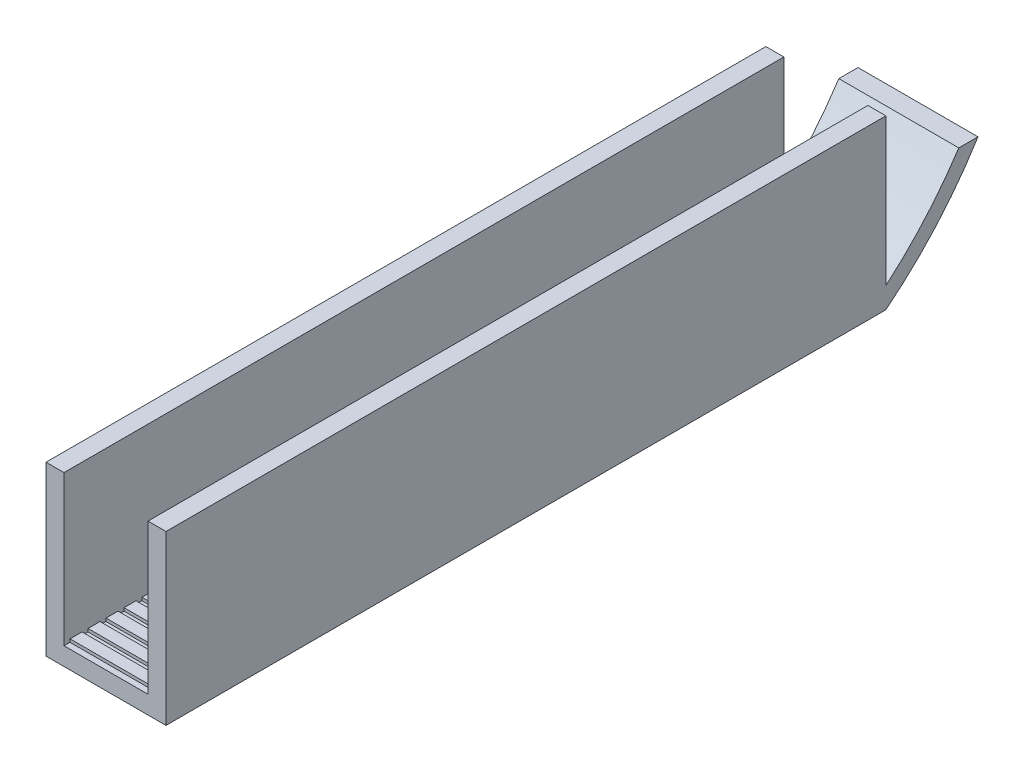
SolidWorks part; units mm, degrees
ref_plane "Front" through (0, 0, 0) normal (0, 0, 1) x (1, 0, 0)
ref_plane "Top" through (0, 0, 0) normal (0, 1, 0) x (1, 0, 0)
ref_plane "Right" through (0, 0, 0) normal (1, 0, 0) x (0, 0, -1)
sketch "Sketch1" plane through (0, 0, 0) normal (0, 0, 1) x (1, 0, 0)
  line L1 (0, 0) -> (-200, 0)
  line L2 (0, 0) -> (0, 30)
  line L3 (0, 30) -> (-200, 30)
  line L4 (-200, 0) -> (-200, 30)
  dimension "D1" = 200
  dimension "D2" = 30
extrude "Boss-Extrude1" add sketch "Sketch1" along normal blind 1200
sketch "Sketch2" plane through (0, 30, 0) normal (0, 1, 0) x (1, 0, 0)
  line L0 (-200, -1200) -> (-200, 0) construction
  line L1 (0, 0) -> (-200, 0)
  line L2 (0, 0) -> (0, -20)
  line L3 (0, -20) -> (-200, -20)
  line L4 (-200, 0) -> (-200, -20)
  line L5 (0, -50) -> (-200, -50)
  line L6 (0, -30) -> (-200, -30)
  line L7 (0, -30) -> (0, -50)
  line L8 (-200, -30) -> (-200, -50)
  line L9 (0, -80) -> (-200, -80)
  line L10 (0, -60) -> (-200, -60)
  line L11 (0, -60) -> (0, -80)
  line L12 (-200, -60) -> (-200, -80)
  line L13 (0, -110) -> (-200, -110)
  line L14 (0, -90) -> (-200, -90)
  line L15 (0, -90) -> (0, -110)
  line L16 (-200, -90) -> (-200, -110)
  line L17 (0, -140) -> (-200, -140)
  line L18 (0, -120) -> (-200, -120)
  line L19 (0, -120) -> (0, -140)
  line L20 (-200, -120) -> (-200, -140)
  line L21 (0, -170) -> (-200, -170)
  line L22 (0, -150) -> (-200, -150)
  line L23 (0, -150) -> (0, -170)
  line L24 (-200, -150) -> (-200, -170)
  line L25 (0, -200) -> (-200, -200)
  line L26 (0, -180) -> (-200, -180)
  line L27 (0, -180) -> (0, -200)
  line L28 (-200, -180) -> (-200, -200)
  line L29 (0, -230) -> (-200, -230)
  line L30 (0, -210) -> (-200, -210)
  line L31 (0, -210) -> (0, -230)
  line L32 (-200, -210) -> (-200, -230)
  line L33 (0, -260) -> (-200, -260)
  line L34 (0, -240) -> (-200, -240)
  line L35 (0, -240) -> (0, -260)
  line L36 (-200, -240) -> (-200, -260)
  line L37 (0, -290) -> (-200, -290)
  line L38 (0, -270) -> (-200, -270)
  line L39 (0, -270) -> (0, -290)
  line L40 (-200, -270) -> (-200, -290)
  line L41 (0, -320) -> (-200, -320)
  line L42 (0, -300) -> (-200, -300)
  line L43 (0, -300) -> (0, -320)
  line L44 (-200, -300) -> (-200, -320)
  line L45 (0, -350) -> (-200, -350)
  line L46 (0, -330) -> (-200, -330)
  line L47 (0, -330) -> (0, -350)
  line L48 (-200, -330) -> (-200, -350)
  line L49 (0, -380) -> (-200, -380)
  line L50 (0, -360) -> (-200, -360)
  line L51 (0, -360) -> (0, -380)
  line L52 (-200, -360) -> (-200, -380)
  line L53 (0, -410) -> (-200, -410)
  line L54 (0, -390) -> (-200, -390)
  line L55 (0, -390) -> (0, -410)
  line L56 (-200, -390) -> (-200, -410)
  line L57 (0, -440) -> (-200, -440)
  line L58 (0, -420) -> (-200, -420)
  line L59 (0, -420) -> (0, -440)
  line L60 (-200, -420) -> (-200, -440)
  line L61 (0, -470) -> (-200, -470)
  line L62 (0, -450) -> (-200, -450)
  line L63 (0, -450) -> (0, -470)
  line L64 (-200, -450) -> (-200, -470)
  line L65 (0, -500) -> (-200, -500)
  line L66 (0, -480) -> (-200, -480)
  line L67 (0, -480) -> (0, -500)
  line L68 (-200, -480) -> (-200, -500)
  line L69 (0, -530) -> (-200, -530)
  line L70 (-200, -510) -> (-200, -530)
  line L71 (0, -510) -> (-200, -510)
  line L72 (0, -510) -> (0, -530)
  line L73 (0, -560) -> (-200, -560)
  line L74 (-200, -540) -> (-200, -560)
  line L75 (0, -540) -> (-200, -540)
  line L76 (0, -540) -> (0, -560)
  line L77 (0, -590) -> (-200, -590)
  line L78 (-200, -570) -> (-200, -590)
  line L79 (0, -570) -> (-200, -570)
  line L80 (0, -570) -> (0, -590)
  line L81 (0, -620) -> (-200, -620)
  line L82 (-200, -600) -> (-200, -620)
  line L83 (0, -600) -> (-200, -600)
  line L84 (0, -600) -> (0, -620)
  line L85 (0, -650) -> (-200, -650)
  line L86 (-200, -630) -> (-200, -650)
  line L87 (0, -630) -> (-200, -630)
  line L88 (0, -630) -> (0, -650)
  line L89 (0, -680) -> (-200, -680)
  line L90 (-200, -660) -> (-200, -680)
  line L91 (0, -660) -> (-200, -660)
  line L92 (0, -660) -> (0, -680)
  line L93 (0, -710) -> (-200, -710)
  line L94 (-200, -690) -> (-200, -710)
  line L95 (0, -690) -> (-200, -690)
  line L96 (0, -690) -> (0, -710)
  line L97 (0, -740) -> (-200, -740)
  line L98 (-200, -720) -> (-200, -740)
  line L99 (0, -720) -> (-200, -720)
  line L100 (0, -720) -> (0, -740)
  line L101 (0, -770) -> (-200, -770)
  line L102 (-200, -750) -> (-200, -770)
  line L103 (0, -750) -> (-200, -750)
  line L104 (0, -750) -> (0, -770)
  line L105 (0, -800) -> (-200, -800)
  line L106 (-200, -780) -> (-200, -800)
  line L107 (0, -780) -> (-200, -780)
  line L108 (0, -780) -> (0, -800)
  line L109 (0, -830) -> (-200, -830)
  line L110 (-200, -810) -> (-200, -830)
  line L111 (0, -810) -> (-200, -810)
  line L112 (0, -810) -> (0, -830)
  line L113 (0, -860) -> (-200, -860)
  line L114 (-200, -840) -> (-200, -860)
  line L115 (0, -840) -> (-200, -840)
  line L116 (0, -840) -> (0, -860)
  line L117 (0, -890) -> (-200, -890)
  line L118 (-200, -870) -> (-200, -890)
  line L119 (0, -870) -> (-200, -870)
  line L120 (0, -870) -> (0, -890)
  line L121 (0, -920) -> (-200, -920)
  line L122 (-200, -900) -> (-200, -920)
  line L123 (0, -900) -> (-200, -900)
  line L124 (0, -900) -> (0, -920)
  line L125 (0, -950) -> (-200, -950)
  line L126 (-200, -930) -> (-200, -950)
  line L127 (0, -930) -> (-200, -930)
  line L128 (0, -930) -> (0, -950)
  line L129 (0, -980) -> (-200, -980)
  line L130 (-200, -960) -> (-200, -980)
  line L131 (0, -960) -> (-200, -960)
  line L132 (0, -960) -> (0, -980)
  line L133 (0, -1010) -> (-200, -1010)
  line L134 (-200, -990) -> (-200, -1010)
  line L135 (0, -990) -> (-200, -990)
  line L136 (0, -990) -> (0, -1010)
  line L137 (0, -1040) -> (-200, -1040)
  line L138 (-200, -1020) -> (-200, -1040)
  line L139 (0, -1020) -> (-200, -1020)
  line L140 (0, -1020) -> (0, -1040)
  line L141 (0, -1070) -> (-200, -1070)
  line L142 (-200, -1050) -> (-200, -1070)
  line L143 (0, -1050) -> (-200, -1050)
  line L144 (0, -1050) -> (0, -1070)
  line L145 (0, -1100) -> (-200, -1100)
  line L146 (-200, -1080) -> (-200, -1100)
  line L147 (0, -1080) -> (-200, -1080)
  line L148 (0, -1080) -> (0, -1100)
  line L149 (0, -1130) -> (-200, -1130)
  line L150 (-200, -1110) -> (-200, -1130)
  line L151 (0, -1110) -> (-200, -1110)
  line L152 (0, -1110) -> (0, -1130)
  line L153 (0, -1160) -> (-200, -1160)
  line L154 (-200, -1140) -> (-200, -1160)
  line L155 (0, -1140) -> (-200, -1140)
  line L156 (0, -1140) -> (0, -1160)
  line L157 (0, -1190) -> (-200, -1190)
  line L158 (-200, -1170) -> (-200, -1190)
  line L159 (0, -1170) -> (-200, -1170)
  line L160 (0, -1170) -> (0, -1190)
  dimension "D1" = 20
  dimension "D2" = 17
  dimension "D3" = 11
  dimension "D4" = 14
extrude "Boss-Extrude2" add sketch "Sketch2" along normal blind 5
sketch "Sketch3" plane through (0, 0, 0) normal (1, 0, 0) x (0, 0, -1)
  line L0 (121.5352, 172.9572) -> (153.5475, 172.9572)
  line L1 (-44.8248, 0) -> (0, 0)
  line L2 (-1200, 0) -> (0, 0) construction
  arc A0 (-44.8248, 0) -> (121.5352, 172.9572) centre (-422.0607, 529.3326) ccw
  arc A1 (0, 0) -> (153.5475, 172.9572) centre (-422.0607, 529.3326) ccw
  dimension "D1" = 1300
extrude "Boss-Extrude3" add sketch "Sketch3" against normal up to surface (200 mm away) up to face at (-200, 32.0988, 602.4691)
sketch "Sketch5" plane through (0, 30, 0) normal (0, 1, 0) x (1, 0, 0)
  line L0 (0, 0) -> (-200, 0) construction
  line L1 (-200, -1200) -> (-170, -1200)
  line L2 (-200, -1200) -> (-200, 0)
  line L3 (-200, 0) -> (-170, 0)
  line L4 (-170, -1200) -> (-170, 0)
  line L6 (0, 0) -> (-30, 0)
  line L7 (0, 0) -> (0, -1200)
  line L8 (0, -1200) -> (-30, -1200)
  line L9 (-30, 0) -> (-30, -1200)
  line L10 (0, -1200) -> (-200, -1200) construction
  point P14 (-185, -1200)
  dimension "D1" = 30
  dimension "D2" = 30
extrude "Boss-Extrude5" add sketch "Sketch5" along normal blind 250
